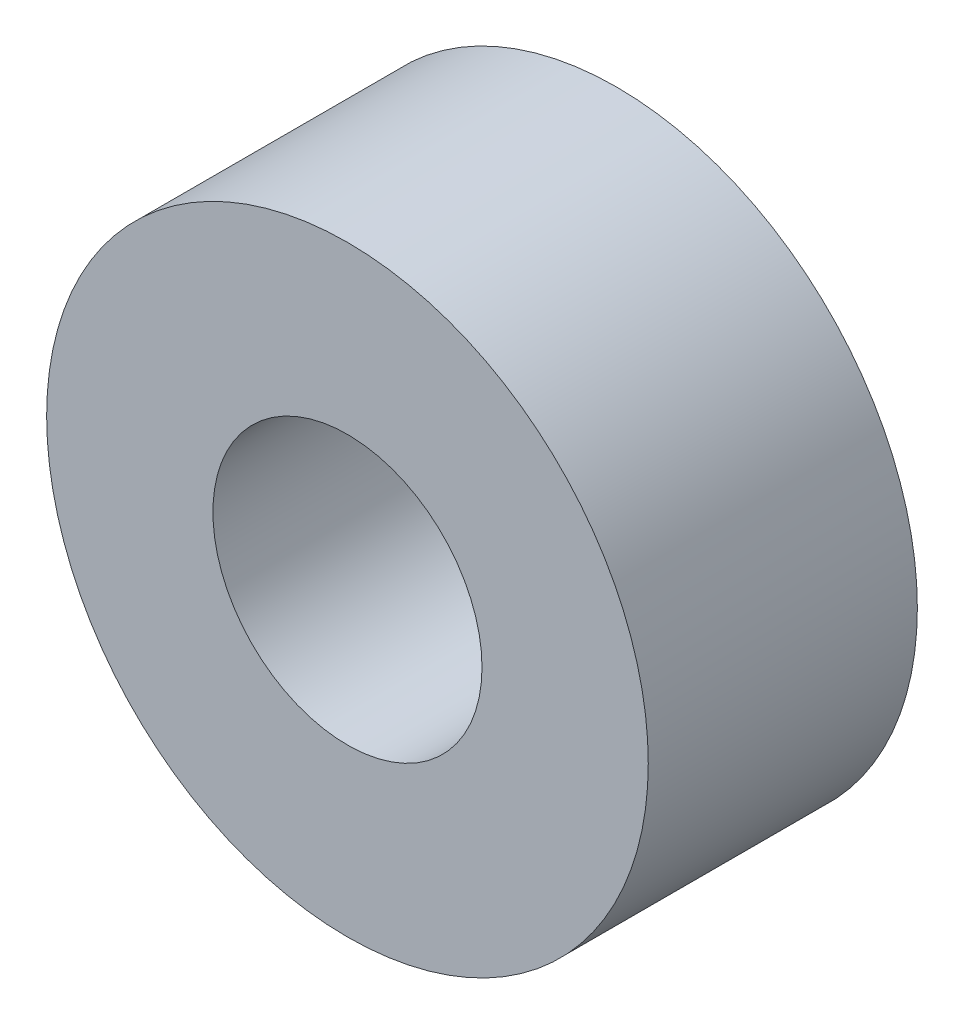
SolidWorks part; units mm, degrees
ref_plane "Front Plane" through (0, 0, 0) normal (0, 0, 1) x (1, 0, 0)
ref_plane "Top Plane" through (0, 0, 0) normal (0, 1, 0) x (1, 0, 0)
ref_plane "Right Plane" through (0, 0, 0) normal (1, 0, 0) x (0, 0, -1)
sketch "Sketch1" plane through (0, 0, 0) normal (0, 0, 1) x (1, 0, 0)
  circle A0 centre (0, 0) radius 5.5896
  circle A1 centre (0, 0) radius 2.5
  dimension "D1" = 5
extrude "Boss-Extrude1" add sketch "Sketch1" along normal blind 5
